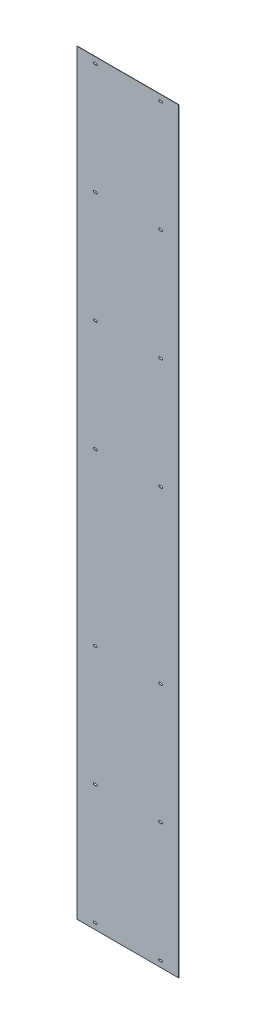
from build123d import *

# Parameters (mm, degrees)
SKETCH_1_W             = 322
SKETCH_1_H             = 2394
EXTRUDE_1_DEPTH        = 0.8
CUT_EXTRUDE_3001_DEPTH = 10


with BuildPart() as part:
    # 草图1 → 凸台-拉伸1 (new body)
    with BuildSketch(Plane.XY):
        Rectangle(SKETCH_1_W, SKETCH_1_H)
    extrude(amount=EXTRUDE_1_DEPTH)

    # 草图2 → 3001 (cut)
    with BuildSketch(Plane.XY.offset(0.8)):
        with BuildLine():
            Line((-106.5, 124), (-100.5, 124))
            ThreePointArc((-100.5, 124), (-97.5, 121), (-100.5, 118))
            Line((-100.5, 118), (-106.5, 118))
            ThreePointArc((-106.5, 118), (-109.5, 121), (-106.5, 124))
        make_face()
        with BuildLine():
            Line((-106.5, 1181), (-100.5, 1181))
            ThreePointArc((-100.5, 1181), (-97.5, 1178), (-100.5, 1175))
            Line((-100.5, 1175), (-106.5, 1175))
            ThreePointArc((-106.5, 1175), (-109.5, 1178), (-106.5, 1181))
        make_face()
        with BuildLine():
            Line((-106.5, 828.666666667), (-100.5, 828.666666667))
            ThreePointArc((-100.5, 828.666666667), (-97.5, 825.666666667), (-100.5, 822.666666667))
            Line((-100.5, 822.666666667), (-106.5, 822.666666667))
            ThreePointArc((-106.5, 822.666666667), (-109.5, 825.666666667), (-106.5, 828.666666667))
        make_face()
        with BuildLine():
            Line((-106.5, -1175), (-100.5, -1175))
            ThreePointArc((-100.5, -1175), (-97.5, -1178), (-100.5, -1181))
            Line((-100.5, -1181), (-106.5, -1181))
            ThreePointArc((-106.5, -1181), (-109.5, -1178), (-106.5, -1175))
        make_face()
        with BuildLine():
            Line((-106.5, 476.333333333), (-100.5, 476.333333333))
            ThreePointArc((-100.5, 476.333333333), (-97.5, 473.333333333), (-100.5, 470.333333333))
            Line((-100.5, 470.333333333), (-106.5, 470.333333333))
            ThreePointArc((-106.5, 470.333333333), (-109.5, 473.333333333), (-106.5, 476.333333333))
        make_face()
        with BuildLine():
            Line((-106.5, -795.5), (-100.5, -795.5))
            ThreePointArc((-100.5, -795.5), (-97.5, -798.5), (-100.5, -801.5))
            Line((-100.5, -801.5), (-106.5, -801.5))
            ThreePointArc((-106.5, -801.5), (-109.5, -798.5), (-106.5, -795.5))
        make_face()
        with BuildLine():
            Line((-106.5, -416), (-100.5, -416))
            ThreePointArc((-100.5, -416), (-97.5, -419), (-100.5, -422))
            Line((-100.5, -422), (-106.5, -422))
            ThreePointArc((-106.5, -422), (-109.5, -419), (-106.5, -416))
        make_face()
        with BuildLine():
            Line((106.5, -1175), (100.5, -1175))
            ThreePointArc((100.5, -1175), (97.5, -1178), (100.5, -1181))
            Line((100.5, -1181), (106.5, -1181))
            ThreePointArc((106.5, -1181), (109.5, -1178), (106.5, -1175))
        make_face()
        with BuildLine():
            Line((106.5, -795.5), (100.5, -795.5))
            ThreePointArc((100.5, -795.5), (97.5, -798.5), (100.5, -801.5))
            Line((100.5, -801.5), (106.5, -801.5))
            ThreePointArc((106.5, -801.5), (109.5, -798.5), (106.5, -795.5))
        make_face()
        with BuildLine():
            Line((106.5, -416), (100.5, -416))
            ThreePointArc((100.5, -416), (97.5, -419), (100.5, -422))
            Line((100.5, -422), (106.5, -422))
            ThreePointArc((106.5, -422), (109.5, -419), (106.5, -416))
        make_face()
        with BuildLine():
            Line((106.5, 476.333333333), (100.5, 476.333333333))
            ThreePointArc((100.5, 476.333333333), (97.5, 473.333333333), (100.5, 470.333333333))
            Line((100.5, 470.333333333), (106.5, 470.333333333))
            ThreePointArc((106.5, 470.333333333), (109.5, 473.333333333), (106.5, 476.333333333))
        make_face()
        with BuildLine():
            Line((106.5, 828.666666667), (100.5, 828.666666667))
            ThreePointArc((100.5, 828.666666667), (97.5, 825.666666667), (100.5, 822.666666667))
            Line((100.5, 822.666666667), (106.5, 822.666666667))
            ThreePointArc((106.5, 822.666666667), (109.5, 825.666666667), (106.5, 828.666666667))
        make_face()
        with BuildLine():
            Line((106.5, 1181), (100.5, 1181))
            ThreePointArc((100.5, 1181), (97.5, 1178), (100.5, 1175))
            Line((100.5, 1175), (106.5, 1175))
            ThreePointArc((106.5, 1175), (109.5, 1178), (106.5, 1181))
        make_face()
        with BuildLine():
            Line((106.5, 124), (100.5, 124))
            ThreePointArc((100.5, 124), (97.5, 121), (100.5, 118))
            Line((100.5, 118), (106.5, 118))
            ThreePointArc((106.5, 118), (109.5, 121), (106.5, 124))
        make_face()
    extrude(amount=-CUT_EXTRUDE_3001_DEPTH, mode=Mode.SUBTRACT)


solid = part.part
